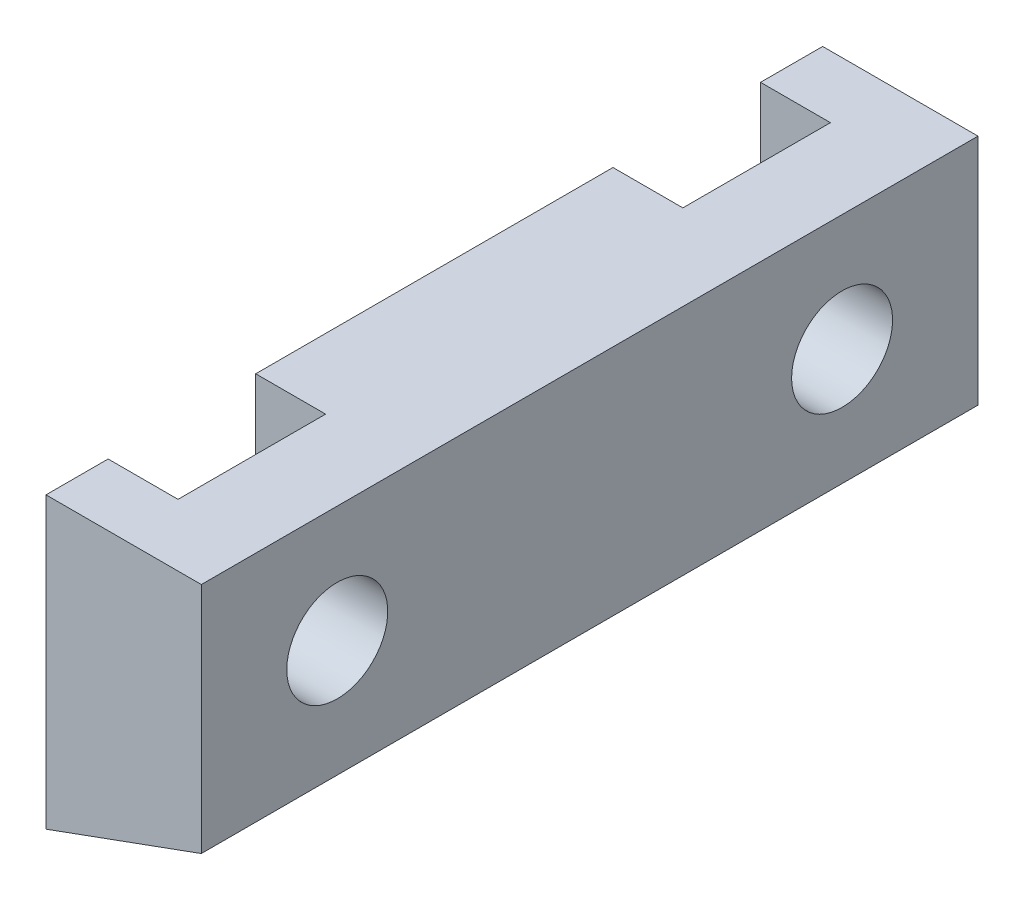
from build123d import *

# Parameters (mm, degrees)
BOSS_EXTRUDE1_DEPTH = 100
SKETCH3_W           = 38
SKETCH3_H           = 122.430323754
CUT_EXTRUDE1_DEPTH  = 18
SKETCH4_R           = 13
CUT_EXTRUDE2_DEPTH  = 60


with BuildPart() as part:
    # Sketch2 → Boss-Extrude1 (new, symmetric)
    with BuildSketch(Plane.XY):
        Polygon((0, 0), (0, 74.558809371), (40, 74.558809371), (40, 14.558809371), align=None)
    extrude(amount=BOSS_EXTRUDE1_DEPTH, both=True)

    # Sketch3 → Cut-Extrude1 (cut)
    with BuildSketch(Plane.ZY):
        with Locations((-65, 44.558809371)):
            Rectangle(SKETCH3_W, SKETCH3_H)
    cut_extrude1 = extrude(amount=-CUT_EXTRUDE1_DEPTH, mode=Mode.SUBTRACT)

    # Mirror1: Cut-Extrude1 across plane
    add(cut_extrude1.mirror(Plane.XY), mode=Mode.SUBTRACT)

    # Sketch4 → Cut-Extrude2 (cut)
    with BuildSketch(Plane(origin=(0, 0, 0), x_dir=(0, 0, -1), z_dir=(1, 0, 0))):
        with Locations(Location((65, 44.558809371, 0), (0, 0, 180))):
            Circle(SKETCH4_R)
        with Locations(Location((-65, 44.558809371, 0), (0, 0, 180))):
            Circle(SKETCH4_R)
    extrude(amount=CUT_EXTRUDE2_DEPTH, mode=Mode.SUBTRACT)


solid = part.part
